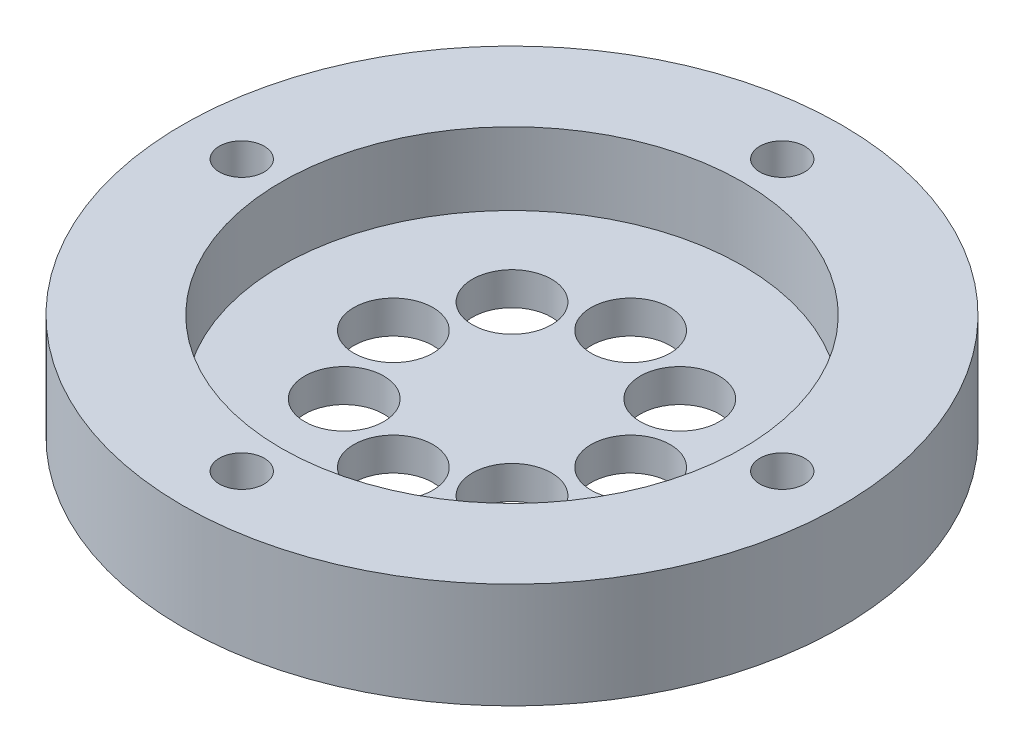
from build123d import *

# Parameters (mm, degrees)
SKETCH1_R                                       = 25
BOSS_EXTRUDE1_DEPTH                             = 8
SKETCH2_R                                       = 17.5
CUT_EXTRUDE1_DEPTH                              = 5.5
SKETCH3_R                                       = 3
CUT_EXTRUDE2_DEPTH                              = 4
CSK_FOR_M3_FLAT_HEAD_MACHINE_SCREW1_D           = 3.4
CSK_FOR_M3_FLAT_HEAD_MACHINE_SCREW1_CSINK_D     = 6.3
CSK_FOR_M3_FLAT_HEAD_MACHINE_SCREW1_CSINK_ANGLE = 90


with BuildPart() as part:
    # Sketch1 → Boss-Extrude1 (new body)
    with BuildSketch(Plane(origin=(0, 0, 0), x_dir=(1, 0, 0), z_dir=(0, 1, 0))):
        with Locations(Location((0, 0, 0), (0, 0, 270))):
            Circle(SKETCH1_R)
    extrude(amount=BOSS_EXTRUDE1_DEPTH)

    # Sketch2 → Cut-Extrude1 (cut)
    with BuildSketch(Plane(origin=(0, 8, 0), x_dir=(1, 0, 0), z_dir=(0, 1, 0))):
        with Locations(Location((0, 0, 0), (0, 0, 270))):
            Circle(SKETCH2_R)
    extrude(amount=-CUT_EXTRUDE1_DEPTH, mode=Mode.SUBTRACT)

    # Sketch3 → Cut-Extrude2 (cut)
    with BuildSketch(Plane.XZ):
        with Locations(Location((0, -9, 0), (0, 0, 270))):
            Circle(SKETCH3_R)
        with Locations(Location((-6.363961031, -6.363961031, 0), (0, 0, 270))):
            Circle(SKETCH3_R)
        with Locations(Location((-9, 0, 0), (0, 0, 270))):
            Circle(SKETCH3_R)
        with Locations(Location((-6.363961031, 6.363961031, 0), (0, 0, 270))):
            Circle(SKETCH3_R)
        with Locations(Location((0, 9, 0), (0, 0, 270))):
            Circle(SKETCH3_R)
        with Locations(Location((6.363961031, 6.363961031, 0), (0, 0, 270))):
            Circle(SKETCH3_R)
        with Locations(Location((9, 0, 0), (0, 0, 270))):
            Circle(SKETCH3_R)
        with Locations(Location((6.363961031, -6.363961031, 0), (0, 0, 270))):
            Circle(SKETCH3_R)
    extrude(amount=-CUT_EXTRUDE2_DEPTH, mode=Mode.SUBTRACT)

    # CSK for M3 Flat Head Machine Screw1 (through all)
    with Locations(Plane(origin=(0, 0, 0), x_dir=(-1, 0, 0), z_dir=(0, -1, 0))):
        with Locations((20.5, 0), (0, 20.5), (-20.5, 0), (0, -20.5)):
            CounterSinkHole(CSK_FOR_M3_FLAT_HEAD_MACHINE_SCREW1_D / 2, CSK_FOR_M3_FLAT_HEAD_MACHINE_SCREW1_CSINK_D / 2, counter_sink_angle=CSK_FOR_M3_FLAT_HEAD_MACHINE_SCREW1_CSINK_ANGLE)


solid = part.part
